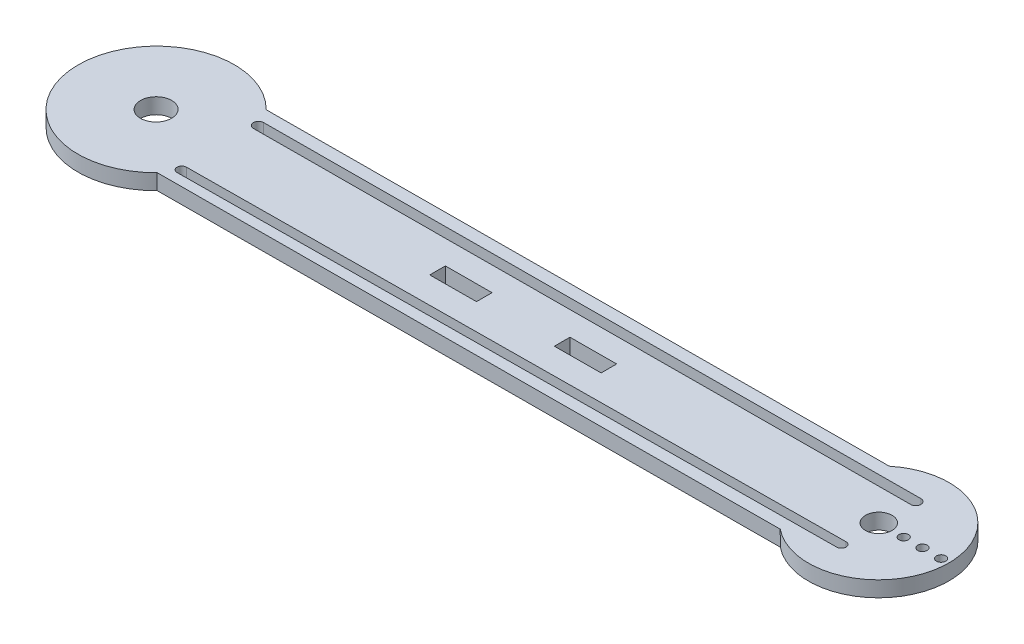
from build123d import *

# Parameters (mm, degrees)
SKETCH_1_R          = 4.25
SKETCH_1_R_2        = 5
EXTRUDE_1_DEPTH     = 5
SKETCH_2_R          = 4.25
SKETCH_2_R_2        = 1.5
CUT_EXTRUDE_1_DEPTH = 10
CUT_EXTRUDE_2_DEPTH = 10
SKETCH_4_W          = 15
SKETCH_4_H          = 5
CUT_EXTRUDE_3_DEPTH = 10


with BuildPart() as part:
    # 草图1 → 凸台-拉伸1 (new body)
    with BuildSketch(Plane(origin=(-1.457577728, 322.176633369, 0), x_dir=(0.9999897661580252, 0.004524110875991417, 0), z_dir=(0.004524110875991416, -0.999989766158025, 0))):
        with BuildLine():
            Line((87.077297431, 423.813689202), (-112.922702569, 423.813689202))
            ThreePointArc((-112.922702569, 423.813689202), (-155.776273641, 406.313689202), (-112.922702569, 388.813689202))
            Line((-112.922702569, 388.813689202), (87.077297431, 388.813689202))
            ThreePointArc((87.077297431, 388.813689202), (123.719433055, 406.313689202), (87.077297431, 423.813689202))
        make_face()
        with Locations((101.219433055, 406.313689202)):
            Circle(SKETCH_1_R, mode=Mode.SUBTRACT)
        with Locations((-130.776273641, 406.313689202)):
            Circle(SKETCH_1_R_2, mode=Mode.SUBTRACT)
    extrude(amount=EXTRUDE_1_DEPTH)

    # 草图2 → 切除-拉伸1 (cut)
    with BuildSketch(Plane(origin=(-1.457577728, 322.176633369, 0), x_dir=(0.9999897661580252, 0.004524110875991416, 0), z_dir=(-0.004524110875991415, 0.999989766158025, 0))):
        with Locations((101.219433055, -406.313689202)):
            Circle(SKETCH_2_R)
        with Locations(Location((121.219433055, -406.313689202, 0), (0, 0, 180))):
            Circle(SKETCH_2_R_2)
        with Locations(Location((115.219433055, -406.313689202, 0), (0, 0, 180))):
            Circle(SKETCH_2_R_2)
        with Locations(Location((109.219433055, -406.313689202, 0), (0, 0, 180))):
            Circle(SKETCH_2_R_2)
        with Locations((-41.214218621, -347.791207337)):
            Circle(SKETCH_2_R_2)
        with Locations((-45.456859308, -343.54856665)):
            Circle(SKETCH_2_R_2)
        with Locations((-49.699499995, -339.305925963)):
            Circle(SKETCH_2_R_2)
        with Locations((-114.690511434, -191.551626966)):
            Circle(SKETCH_2_R_2)
        with Locations((-114.690511434, -185.551626966)):
            Circle(SKETCH_2_R_2)
        with Locations((-114.690511434, -179.551626966)):
            Circle(SKETCH_2_R_2)
        with Locations((-56.168029569, -29.117975291)):
            Circle(SKETCH_2_R_2)
        with Locations((-51.925388882, -24.875334604)):
            Circle(SKETCH_2_R_2)
        with Locations((-47.682748195, -20.632693917)):
            Circle(SKETCH_2_R_2)
        with Locations((100.071550802, 44.358317523)):
            Circle(SKETCH_2_R_2)
        with Locations((106.071550802, 44.358317523)):
            Circle(SKETCH_2_R_2)
        with Locations((112.071550802, 44.358317523)):
            Circle(SKETCH_2_R_2)
        with Locations((262.505202477, -14.164164342)):
            Circle(SKETCH_2_R_2)
        with Locations((266.747843164, -18.406805029)):
            Circle(SKETCH_2_R_2)
        with Locations((270.990483851, -22.649445716)):
            Circle(SKETCH_2_R_2)
        with Locations((335.981495291, -170.403744713)):
            Circle(SKETCH_2_R_2)
        with Locations((335.981495291, -176.403744713)):
            Circle(SKETCH_2_R_2)
        with Locations((335.981495291, -182.403744713)):
            Circle(SKETCH_2_R_2)
        with Locations((277.459013426, -332.837396388)):
            Circle(SKETCH_2_R_2)
        with Locations((273.216372738, -337.080037075)):
            Circle(SKETCH_2_R_2)
        with Locations((268.973732051, -341.322677763)):
            Circle(SKETCH_2_R_2)
    extrude(amount=-CUT_EXTRUDE_1_DEPTH, mode=Mode.SUBTRACT)

    # 草图3 → 切除-拉伸2 (cut)
    with BuildSketch(Plane(origin=(-1.457577728, 322.176633369, 0), x_dir=(0.9999897661580252, 0.004524110875991416, 0), z_dir=(-0.004524110875991415, 0.999989766158025, 0))):
        with BuildLine():
            Line((-109.757857106, -392.813689202), (101.219433055, -392.813689202))
            ThreePointArc((101.219433055, -392.813689202), (102.853546755, -394.447802903), (101.219433055, -396.081916603))
            Line((101.219433055, -396.081916603), (-109.757857106, -396.081916603))
            ThreePointArc((-109.757857106, -396.081916603), (-111.391970807, -394.447802903), (-109.757857106, -392.813689202))
        make_face()
        with BuildLine():
            Line((-109.752317405, -420.592841481), (101.219433055, -419.813689202))
            ThreePointArc((101.219433055, -419.813689202), (102.713883124, -418.30815973), (101.208353652, -416.813709661))
            Line((101.208353652, -416.813709661), (-109.763396807, -417.59286194))
            ThreePointArc((-109.763396807, -417.59286194), (-111.257846876, -419.098391411), (-109.752317405, -420.592841481))
        make_face()
    extrude(amount=-CUT_EXTRUDE_2_DEPTH, mode=Mode.SUBTRACT)

    # 草图4 → 切除-拉伸3 (cut)
    with BuildSketch(Plane(origin=(-1.457577728, 322.176633369, 0), x_dir=(0.9999897661580252, 0.004524110875991416, 0), z_dir=(-0.004524110875991415, 0.999989766158025, 0))):
        with Locations((-32.922702569, -406.313689202)):
            Rectangle(SKETCH_4_W, SKETCH_4_H)
        with Locations((7.077297431, -406.313689202)):
            Rectangle(SKETCH_4_W, SKETCH_4_H)
    extrude(amount=-CUT_EXTRUDE_3_DEPTH, mode=Mode.SUBTRACT)


solid = part.part
